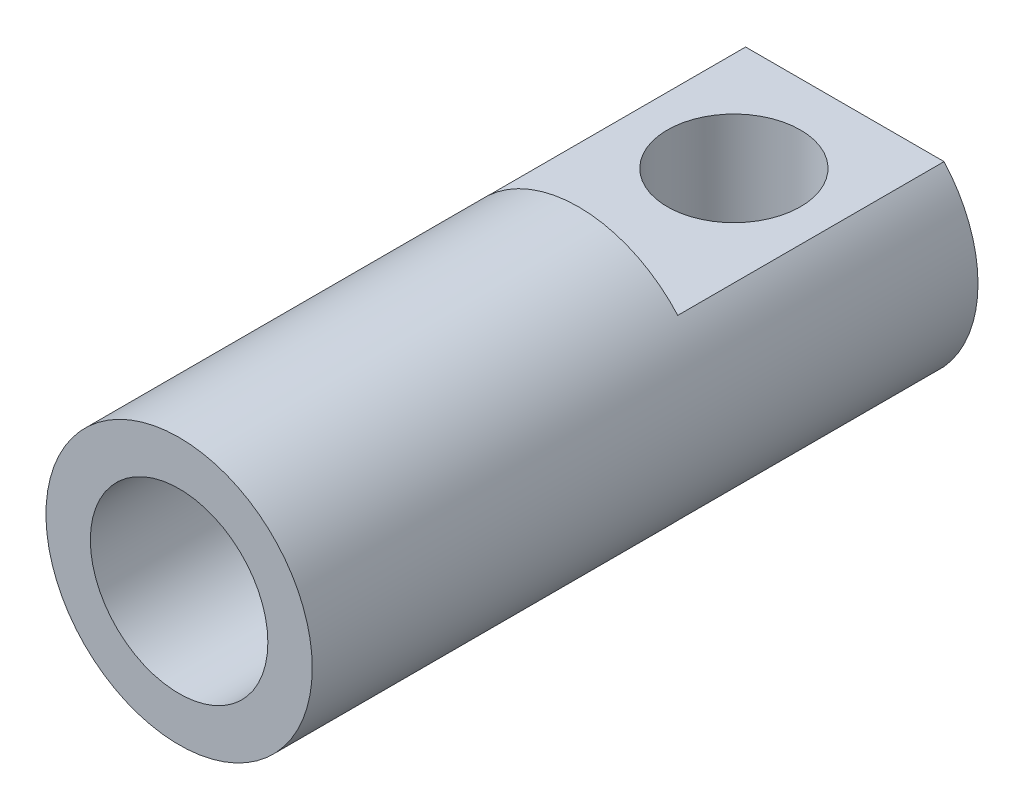
from build123d import *

# Parameters (mm, degrees)
SKETCH1_R               = 6
BOSS_EXTRUDE1_DEPTH     = 30
CUT_EXTRUDE1_START      = -4
SKETCH2_W               = 22.463140108
SKETCH2_H               = 15.309140372
CUT_EXTRUDE1_DEPTH      = 10
CUT_EXTRUDE2_DEPTH      = 33.186953879
CUT_EXTRUDE2_DEPTH_BACK = 33.186953879
SKETCH3_R               = 3
SKETCH4_R               = 4
CUT_EXTRUDE3_DEPTH      = 10


with BuildPart() as part:
    # Sketch1 → Boss-Extrude1 (new body)
    with BuildSketch(Plane.XY):
        Circle(SKETCH1_R)
    extrude(amount=BOSS_EXTRUDE1_DEPTH)

    # Sketch2 → Cut-Extrude1 (cut)
    with BuildSketch(Plane(origin=(0, 0, 0), x_dir=(1, 0, 0), z_dir=(0, 1, 0)).offset(CUT_EXTRUDE1_START)):
        with Locations((0.351673426, -4.345429814)):
            Rectangle(SKETCH2_W, SKETCH2_H)
    cut_extrude1 = extrude(amount=-CUT_EXTRUDE1_DEPTH, mode=Mode.SUBTRACT)

    # Mirror1: Cut-Extrude1 across plane
    add(cut_extrude1.mirror(Plane.ZX), mode=Mode.SUBTRACT)

    # Sketch3 → Cut-Extrude2 (cut, two sides: drawn at the far end of the back side and taken through both)
    with BuildSketch(Plane.XZ.offset(4).offset(-CUT_EXTRUDE2_DEPTH_BACK)):
        with Locations(Location((0, 5, 0), (0, 0, 270))):
            Circle(SKETCH3_R)
    extrude(amount=CUT_EXTRUDE2_DEPTH + CUT_EXTRUDE2_DEPTH_BACK, mode=Mode.SUBTRACT)

    # Sketch4 → Cut-Extrude3 (cut)
    with BuildSketch(Plane.XY.offset(30)):
        Circle(SKETCH4_R)
    extrude(amount=-CUT_EXTRUDE3_DEPTH, mode=Mode.SUBTRACT)


solid = part.part
